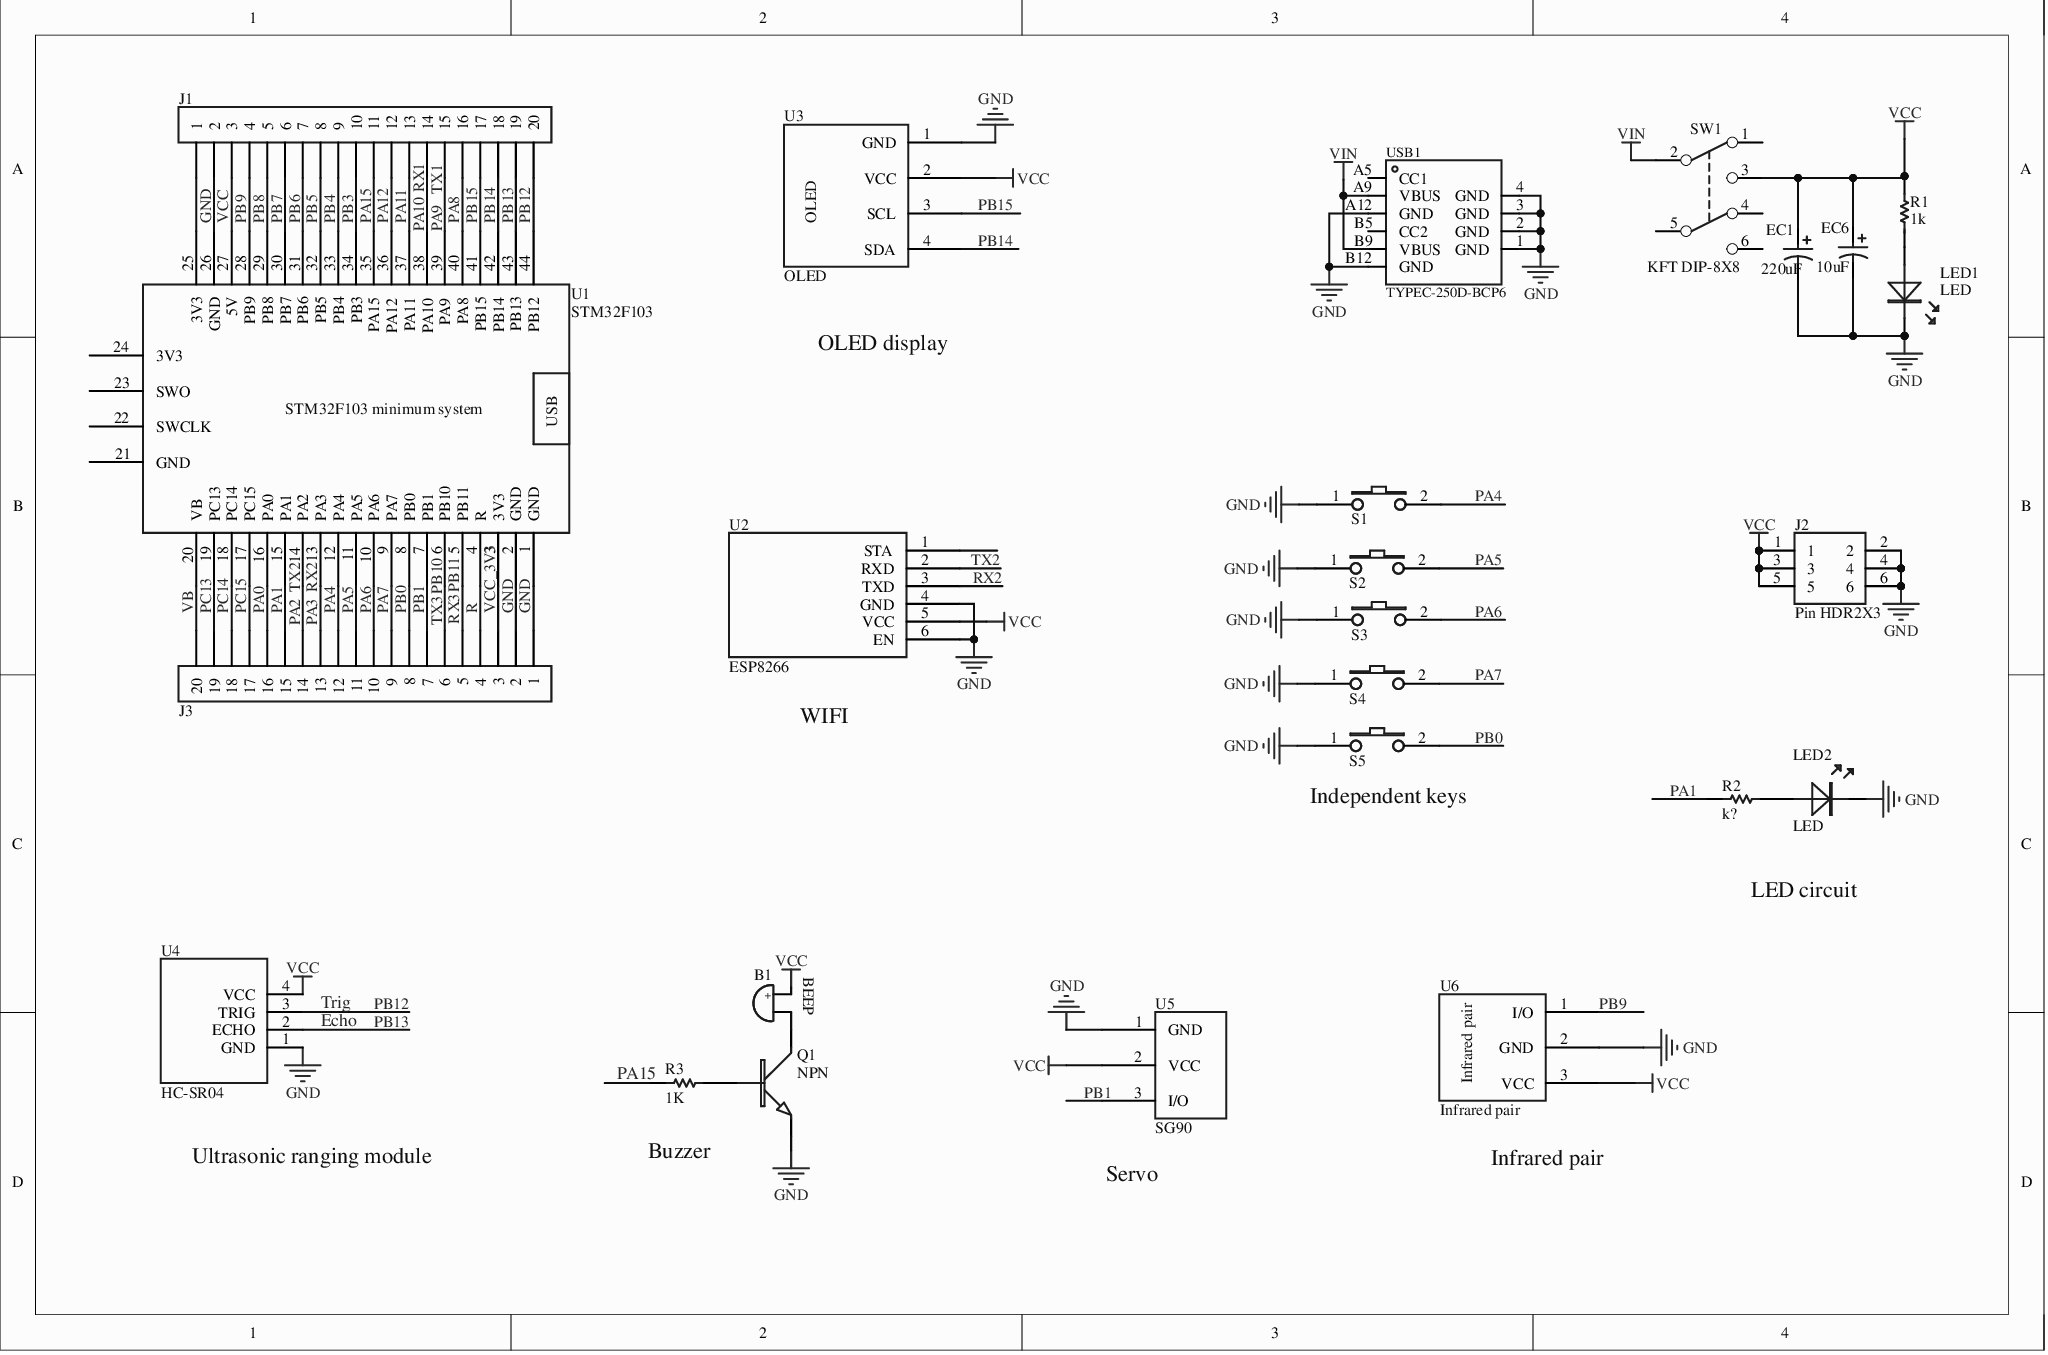
[diagram p0: MISC51211-2.schdoc]
# Altium project MISC51211-3.PrjPcb
1 sheet, 25 parts. Net scope: global (net labels, ports and power ports of the same name join across sheets).
Board file: MISC51211.pcbdoc

## Sheet MISC51211-2.schdoc
size 292 x 193 mm; Name: MISC51211

### Parts
B1  BEEP  [BEEP 7.6X12X7.5]
EC1  220uF  [DIP-EC2.5X5X11]
EC6  10uF  [DIP-EC2.5X5X11]
J1  (no value)  [Pin HDR1X20/2.54mm-S]
J2  Pin HDR2X3  [Pin HDR2X3/2.54mm-S]
J3  (no value)  [Pin HDR1X20/2.54mm-S]
LED1  LED  [LED5-BLUE]
LED2  LED  [LED5-BLUE]
Q1  NPN  [TO-92A]
R1  1k  [AXIAL0.3]
R2  k?  [AXIAL0.3]
R3  1K  [AXIAL0.3]
S1  BUTTOM  [DIP-6X6X5]  (value not drawn)
S2  BUTTOM  [DIP-6X6X5]  (value not drawn)
S3  BUTTOM  [DIP-6X6X5]  (value not drawn)
S4  BUTTOM  [DIP-6X6X5]  (value not drawn)
S5  BUTTOM  [DIP-6X6X5]  (value not drawn)
SW1  KFT DIP-8X8  [KFT DIP-8X8]
U1  STM32F103  [STM32FF103]
U2  ESP8266  [ECB02]
U3  OLED  [OLED]
U4  HC-SR04  [超声波MODE]
U5  SG90  [SG90]
U6  Infrared pair  [红外对管]
USB1  TYPEC-250D-BCP6  [TYP-C-6]

### Nets
GND: EC1.2 EC6.2 J1.2 J2.2 J2.4 J2.6 J3.1 J3.2 LED1.K LED2.K Q1.E S1.1 S2.1 S3.1 S4.1 S5.1 U1.1(GND) U1.2(GND) U1.26(GND) U2.4(GND) U2.6(EN) U3.1(GND) U4.1(GND) U5.1(GND) U6.2(GND) USB1.1(GND) USB1.2(GND) USB1.3(GND) USB1.4(GND) USB1.A12(GND) USB1.B12(GND)
VCC: B1.1 EC1.1 EC6.1 J1.3 J2.1 J2.3 J2.5 R1.2 SW1.3 U1.27(5V) U2.5(VCC) U3.2(VCC) U4.4(VCC) U5.2(VCC) U6.3(VCC)
VIN: SW1.2 USB1.A9(VBUS) USB1.B9(VBUS)
Echo: J1.19 U1.43(PB13) U4.2(ECHO)  [also labelled PB13]
PA0: J3.16 U1.16(PA0)
PA1: J3.15 R2.1 U1.15(PA1)
PA2: J3.14 U1.14(PA2) U2.2(RXD)  [also labelled TX2]
PA3: J3.13 U1.13(PA3) U2.3(TXD)  [also labelled RX2]
PA4: J3.12 S1.2 U1.12(PA4)
PA5: J3.11 S2.2 U1.11(PA5)
PA6: J3.10 S3.2 U1.10(PA6)
PA7: J3.9 S4.2 U1.9(PA7)
PA8: J1.16 U1.40(PA8)
PA9: J1.15 U1.39(PA9)  [also labelled TX1]
PA10: J1.14 U1.38(PA10)  [also labelled RX1]
PA11: J1.13 U1.37(PA11)
PA12: J1.12 U1.36(PA12)
PA15: J1.11 R3.1 U1.35(PA15)
PB0: J3.8 S5.2 U1.8(PB0)
PB1: J3.7 U1.7(PB1) U5.3(I/O)
PB3: J1.10 U1.34(PB3)
PB4: J1.9 U1.33(PB4)
PB5: J1.8 U1.32(PB5)
PB6: J1.7 U1.31(PB6)
PB7: J1.6 U1.30(PB7)
PB8: J1.5 U1.29(PB8)
PB9: J1.4 U1.28(PB9) U6.1(I/O)
PB10: J3.6 U1.6(PB10)  [also labelled TX3]
PB11: J3.5 U1.5(PB11)  [also labelled RX3]
PB12: J1.20 U1.44(PB12) U4.3(TRIG)  [also labelled Trig]
PB14: J1.18 U1.42(PB14) U3.4(SDA)
PB15: J1.17 U1.41(PB15) U3.3(SCL)
PC13: J3.19 U1.19(PC13)
PC14: J3.18 U1.18(PC14)
PC15: J3.17 U1.17(PC15)
R: J3.4 U1.4(R)
VB: J3.20 U1.20(VB)
VCC_3V3: J3.3 U1.3(3V3)
NetB1_2: B1.2 Q1.C
NetJ1_1: J1.1 U1.25(3V3)
NetLED1_A: LED1.A R1.1
NetLED2_A: LED2.A R2.2
NetQ1_B: Q1.B R3.2

Not connected (* = marked no-connect by the designer): SW1 1 4 5 6; U1 21(GND) 22(SWCLK) 23(SWO) 24(3V3); U2 1(STA); USB1 A5(CC1) B5(CC2)

### Notes on the sheet
- OLED display
- WIFI
- (near S5) Independent keys
- LED circuit
- Ultrasonic ranging module
- (near Q1) Buzzer
- (near U5) Servo
- (near U6) Infrared pair

### Library data of the parts
B1 = BEEP: Buzzer; Origin Footprint: BEEP 6.5x12x6; OriginFootprint 2: BEEP 5x9x5.5; OriginFootprint 3: BEEP 6.5x12x8.5; OriginFootprint 4: BEEP 7.6X12X9.5; UniqueId: ecd4cc2f475f8764; AddInBom: yes; Device: BEEP; DesignItemID: BEEP; LibraryName: Buzzer; SymbolName: BEEP; FootprintName: BEEP 7.6X12X7.5
EC1 = 220uF: Polarized capacitor; Origin Footprint: RB.15/.3; UniqueId: 1f6a804da79fa676; SymbolName: CAP_EC; AddInBom: yes; Device: 220uF; DesignItemID: CAP_EC; LibraryName: Reference; FootprintName: DIP-EC2.5X5X11
EC6 = 10uF: Polarized capacitor; Origin Footprint: RB.15/.3; UniqueId: 360d8aaef8286b78; SymbolName: CAP_EC; AddInBom: yes; Device: 10uF; DesignItemID: CAP_EC; LibraryName: Reference; FootprintName: DIP-EC2.5X5X11
J1 = J1: Origin Footprint: Pin HDR1X20/2.54mm-W; UniqueId: 9f49826860c2c79d; SymbolName: Pin HDR1X20; AddInBom: yes; Device: J1; DesignItemID: Pin HDR1X20; LibraryName: Pin header; FootprintName: Pin HDR1X20/2.54mm-S
J2 = Pin HDR2X3: Origin Footprint: Pin HDR2X3/2.54mm-W; UniqueId: 42913bc3a3449998; AddInBom: yes; Device: Pin HDR2X3; DesignItemID: Pin HDR2X3; LibraryName: Pin header; SymbolName: Pin HDR2X3; FootprintName: Pin HDR2X3/2.54mm-S
J3 = J3: Origin Footprint: Pin HDR1X20/2.54mm-W; UniqueId: 6ca7fcf0d18ad80e; SymbolName: Pin HDR1X20; AddInBom: yes; Device: J3; DesignItemID: Pin HDR1X20; LibraryName: Pin header; FootprintName: Pin HDR1X20/2.54mm-S
LED1 = LED: Origin Footprint: LED5-GRE; OriginFootprint 2: LED5-RED; OriginFootprint 3: LED5-YEL; OriginFootprint 4: LED3-BLUE; OriginFootprint 5: LED3-GRE; OriginFootprint 6: LED3-RED; OriginFootprint 7: LED3-YEL; OriginFootprint 8: 1WLED; OriginFootprint 9: LED-0603B; OriginFootprint 10: LED-0603G; OriginFootprint 11: LED-0805R; OriginFootprint 12: LED-0603W; OriginFootprint 13: LED-0603Y; OriginFootprint 14: LED-0805B; OriginFootprint 15: LED-0805G; OriginFootprint 18: LED-0805Y; OriginFootprint 19: LED-1206B; OriginFootprint 20: LED-1206G; OriginFootprint 21: LED-1206R; OriginFootprint 22: LED-1206W; OriginFootprint 23: LED-1206Y; UniqueId: a4c4b307afb8d999; AddInBom: yes; Device: LED; OriginFootprint 16: LED-0805R; OriginFootprint 17: LED-0603W; DesignItemID: LED; LibraryName: LED; SymbolName: LED; FootprintName: LED5-BLUE
LED2 = LED: Origin Footprint: LED5-GRE; OriginFootprint 2: LED5-RED; OriginFootprint 3: LED5-YEL; OriginFootprint 4: LED3-BLUE; OriginFootprint 5: LED3-GRE; OriginFootprint 6: LED3-RED; OriginFootprint 7: LED3-YEL; OriginFootprint 8: 1WLED; OriginFootprint 9: LED-0603B; OriginFootprint 10: LED-0603G; OriginFootprint 11: LED-0805R; OriginFootprint 12: LED-0603W; OriginFootprint 13: LED-0603Y; OriginFootprint 14: LED-0805B; OriginFootprint 15: LED-0805G; OriginFootprint 18: LED-0805Y; OriginFootprint 19: LED-1206B; OriginFootprint 20: LED-1206G; OriginFootprint 21: LED-1206R; OriginFootprint 22: LED-1206W; OriginFootprint 23: LED-1206Y; UniqueId: a245eb2d2aad9559; AddInBom: yes; Device: LED; OriginFootprint 16: LED-0805R; OriginFootprint 17: LED-0603W; DesignItemID: LED; LibraryName: Display library; SymbolName: LED; FootprintName: LED5-BLUE
Q1 = NPN: NPN transistor; Origin Footprint: SOT-23; OriginFootprint 2: TO126; OriginFootprint 3: TO220A; OriginFootprint 4: TO220B; OriginFootprint 5: TO-92B; UniqueId: 047b734180970fea; AddInBom: yes; Device: NPN; DesignItemID: NPN; LibraryName: Transistor; SymbolName: NPN; FootprintName: TO-92A
R1 = 1k: Origin Footprint: 0201R; OriginFootprint 2: 0402R; OriginFootprint 3: 0603R; OriginFootprint 4: 0805R; OriginFootprint 5: 1206R; OriginFootprint 6: 1812R; OriginFootprint 7: 2010R; OriginFootprint 8: 2512R; OriginFootprint 9: AXIAL0.4; OriginFootprint 10: AXIAL0.5; OriginFootprint 11: AXIAL0.6; OriginFootprint 12: AXIAL0.7; OriginFootprint 13: AXIAL0.9; OriginFootprint 14: AXIAL0.8; OriginFootprint 15: AXIAL1.0; UniqueId: 4e166b190d4de1c3; SymbolName: RES; AddInBom: yes; Device: 1k; DesignItemID: RES; LibraryName: Resistor; FootprintName: AXIAL0.3
R2 = k?: Origin Footprint: 0201R; OriginFootprint 2: 0402R; OriginFootprint 3: 0603R; OriginFootprint 4: 0805R; OriginFootprint 5: 1206R; OriginFootprint 6: 1812R; OriginFootprint 7: 2010R; OriginFootprint 8: 2512R; OriginFootprint 9: AXIAL0.4; OriginFootprint 10: AXIAL0.5; OriginFootprint 11: AXIAL0.6; OriginFootprint 12: AXIAL0.7; OriginFootprint 13: AXIAL0.9; OriginFootprint 14: AXIAL0.8; OriginFootprint 15: AXIAL1.0; UniqueId: 06442d24ab060343; SymbolName: RES; AddInBom: yes; Device: k?; DesignItemID: RES; LibraryName: Resistor; FootprintName: AXIAL0.3
R3 = 1K: Origin Footprint: 0201R; OriginFootprint 2: 0402R; OriginFootprint 3: 0603R; OriginFootprint 4: 0805R; OriginFootprint 5: 1206R; OriginFootprint 6: 1812R; OriginFootprint 7: 2010R; OriginFootprint 8: 2512R; OriginFootprint 9: AXIAL0.4; OriginFootprint 10: AXIAL0.5; OriginFootprint 11: AXIAL0.6; OriginFootprint 12: AXIAL0.7; OriginFootprint 13: AXIAL0.9; OriginFootprint 14: AXIAL0.8; OriginFootprint 15: AXIAL1.0; UniqueId: 6e26aea592918673; SymbolName: RES; AddInBom: yes; Device: 1K; DesignItemID: RES; LibraryName: Resistor; FootprintName: AXIAL0.3
S1 = BUTTOM: Button; UniqueId: da892dff24010eb4; AddInBom: yes; Device: BUTTOM; DesignItemID: BUTTOM; LibraryName: Reference; SymbolName: BUTTOM; FootprintName: DIP-6X6X5
S2 = BUTTOM: Button; UniqueId: b3b756e6393b620b; AddInBom: yes; Device: BUTTOM; DesignItemID: BUTTOM; LibraryName: Reference; SymbolName: BUTTOM; FootprintName: DIP-6X6X5
S3 = BUTTOM: Button; UniqueId: 7b79a888bb89fb64; AddInBom: yes; Device: BUTTOM; DesignItemID: BUTTOM; LibraryName: Reference; SymbolName: BUTTOM; FootprintName: DIP-6X6X5
S4 = BUTTOM: Button; UniqueId: 5bcf7e05ad3bc526; AddInBom: yes; Device: BUTTOM; DesignItemID: BUTTOM; LibraryName: Reference; SymbolName: BUTTOM; FootprintName: DIP-6X6X5
S5 = BUTTOM: Button; UniqueId: 3819b3f665fa52ad; AddInBom: yes; Device: BUTTOM; DesignItemID: BUTTOM; LibraryName: Reference; SymbolName: BUTTOM; FootprintName: DIP-6X6X5
SW1 = KFT DIP-8X8: UniqueId: 1070c7afd779bef2; AddInBom: yes; Device: KFT DIP-8X8; DesignItemID: KFT DIP-8X8; LibraryName: Power switch; SymbolName: KFT DIP-8X8; FootprintName: KFT DIP-8X8
U1 = STM32F103: UniqueId: 48a4a086d8c42a18; AddInBom: yes; Device: STM32F103; DesignItemID: STM32F103; LibraryName: Custom schematic library; Description: STM32F103; SymbolName: STM32F103; FootprintName: STM32FF103
U2 = ESP8266: UniqueId: d74c11912b695046; AddInBom: yes; Device: ESP8266; DesignItemID: ECB02; LibraryName: Sensors; SymbolName: ECB02; FootprintName: ECB02
U3 = OLED: UniqueId: eac3f191c372887e; AddInBom: yes; Device: OLED; DesignItemID: OLED; LibraryName: Custom schematic library; Description: OLED; SymbolName: OLED; FootprintName: OLED
U4 = HC-SR04: Ultrasonic module; UniqueId: e5d1bee62801ccc5; SymbolName: Ultrasonic MODE; AddInBom: yes; ModelId: d459d248281f4140aaafbda3f8c1b0d5; Device: HC-SR04; DesignItemID: 超声波MODE; LibraryName: Reference; FootprintName: Ultrasonic MODE; ModelName: HC-SR04
U5 = SG90: UniqueId: 65fd737caad1a168; AddInBom: yes; Device: SG90; DesignItemID: SG90; LibraryName: Custom schematic library; Description: SG90; SymbolName: SG90; FootprintName: SG90
U6 = 红外对管: UniqueId: cb0a5e759a2bc85d; AddInBom: yes; Device: Infrared pair; DesignItemID: 红外对管; LibraryName: Custom schematic library; Description: Infrared pair; SymbolName: Infrared pair; FootprintName: Infrared pair
USB1 = TYPEC-250D-BCP6: BOM_Manufacturer: XUNPU; Contributor: LCSC; UniqueId: 139325cbc0f4fece; AddInBom: yes; Device: TYPEC-250D-BCP6; BOM_Supplier: LCSC; BOM_Supplier Part: C720626; BOM_Manufacturer Part: TYPEC-250D-BCP6; BOM_JLCPCB Part Class: Extended Part; spicePre: U; spiceSymbolName: TYPEC-250D-BCP6; DesignItemID: TYPEC-250D-BCP6; LibraryName: Power socket; SymbolName: TYPEC-250D-BCP6; FootprintName: TYP-C-6